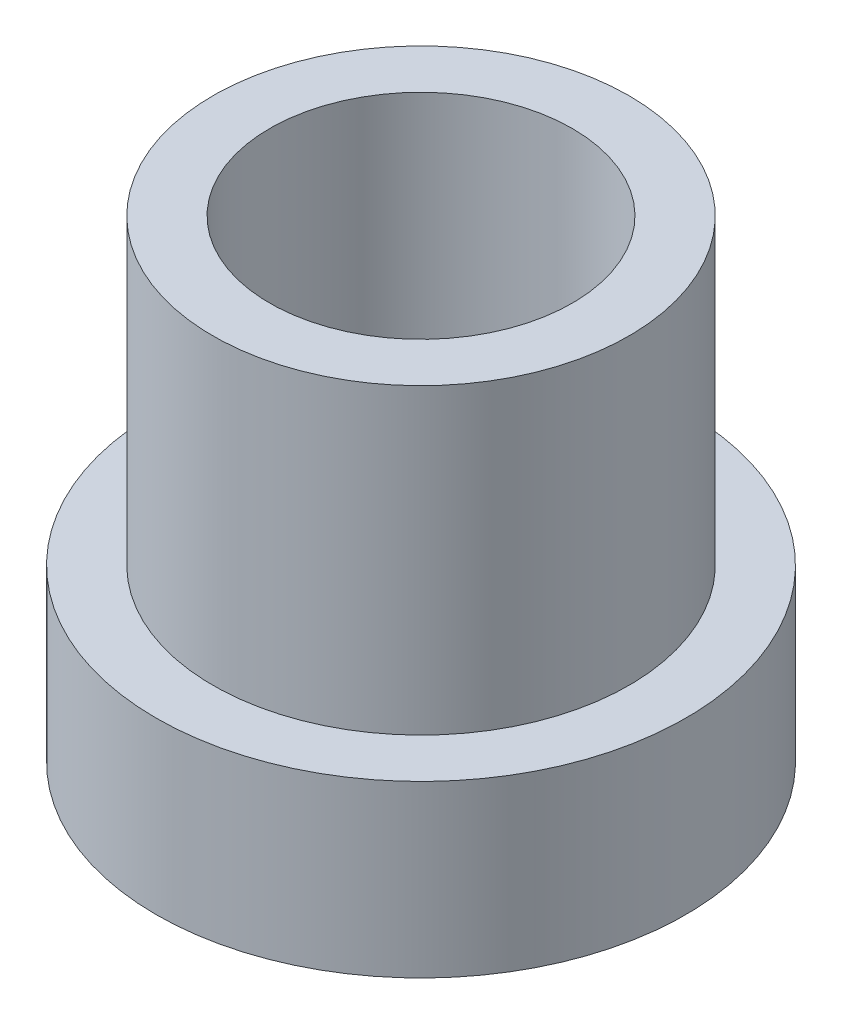
from build123d import *

# Parameters (mm, degrees)
SKETCH_2_R          = 1.5
CUT_EXTRUDE_1_DEPTH = 10


with BuildPart() as part:
    # 草图1 → 旋转1 (revolve)
    with BuildSketch(Plane.XY, mode=Mode.PRIVATE) as revolve_1_sk:
        Polygon((4, 7.261363636), (5.5, 7.261363636), (5.5, -0.738636364), (7, -0.738636364), (7, -5.238636364), (4, -5.238636364), align=None)
    revolve(revolve_1_sk.sketch.rotate(Axis((0, 0, 0), (0, 1, 0)), 90), axis=Axis((0, 0, 0), (0, 1, 0)))

    # 草图2 → 切除-拉伸1 (cut)
    with BuildSketch(Plane.XY):
        with Locations(Location((0, -2.988636364, 0), (0, 0, 270.000000001))):
            Circle(SKETCH_2_R)
    extrude(amount=-CUT_EXTRUDE_1_DEPTH, mode=Mode.SUBTRACT)


solid = part.part
